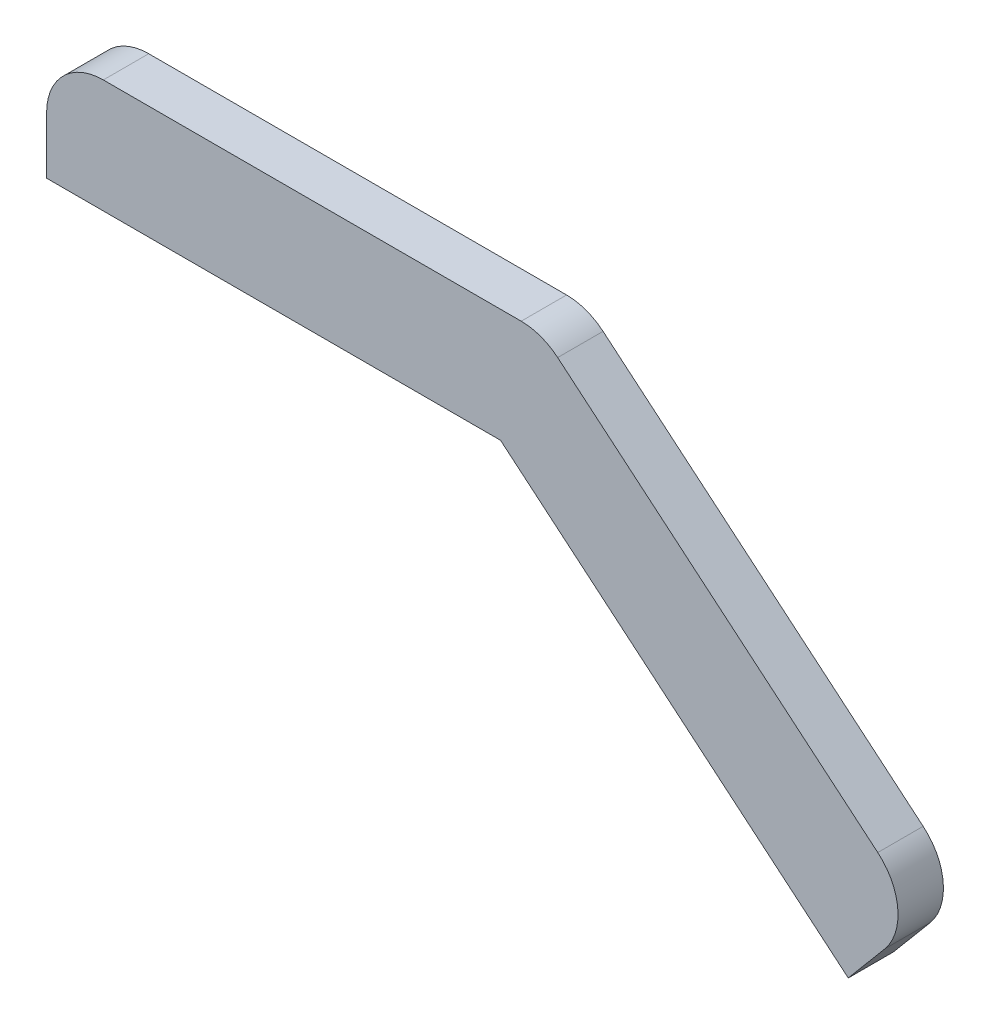
SolidWorks part; units mm, degrees
ref_plane "Front Plane" through (0, 0, 0) normal (0, 0, 1) x (1, 0, 0)
ref_plane "Top Plane" through (0, 0, 0) normal (0, 1, 0) x (1, 0, 0)
ref_plane "Right Plane" through (0, 0, 0) normal (1, 0, 0) x (0, 0, -1)
sketch "Sketch1" plane through (0, 0, 0) normal (0, 0, 1) x (1, 0, 0)
  line L0 (0, 0) -> (80, 0)
  line L1 (80, 0) -> (141.2836, -51.423)
  line L2 (141.2836, -51.423) -> (154.1393, -36.1021)
  line L3 (154.1393, -36.1021) -> (87.2794, 20)
  line L4 (87.2794, 20) -> (0, 20)
  line L5 (0, 20) -> (0, 0)
  dimension "D1" = 80
  dimension "D2" = 80
  dimension "D3" = 20
  dimension "D4" = 20
  dimension "D5" = 140
extrude "Boss-Extrude1" add sketch "Sketch1" along normal blind 8
fillet "Fillet1" radius 10 3 edges at (87.2794, 20, 4) (154.1393, -36.1021, 4) (0, 20, 4)
